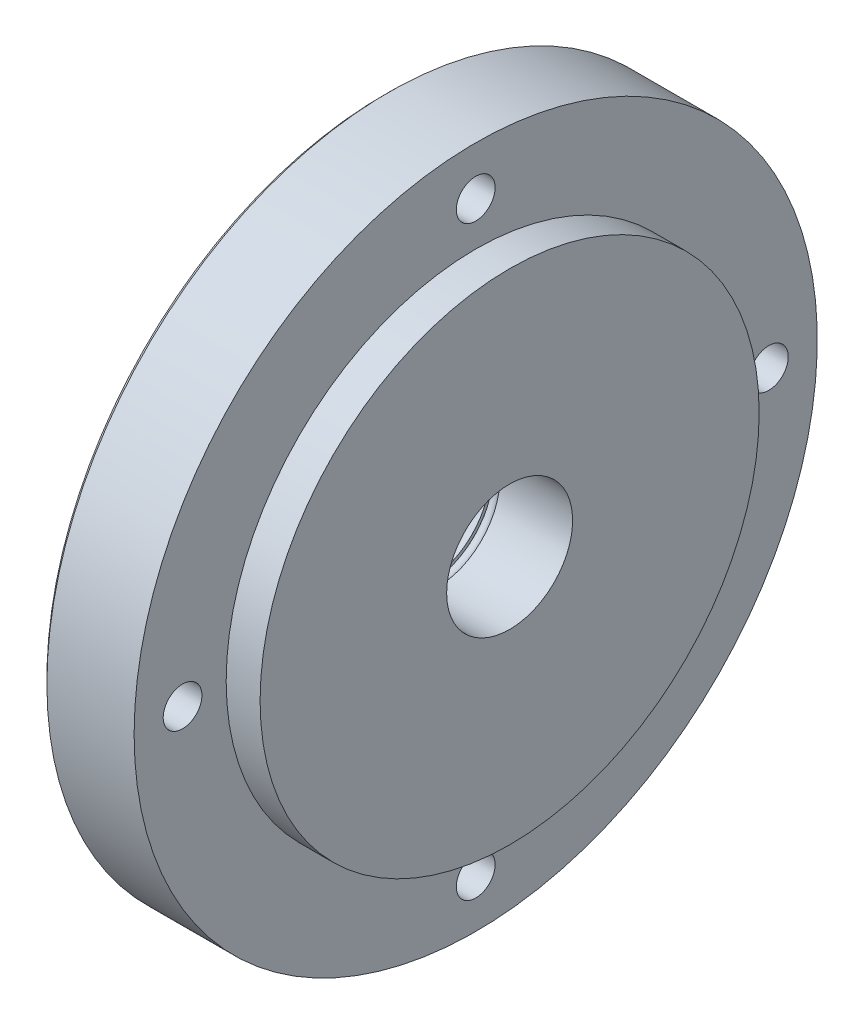
from build123d import *

# Parameters (mm, degrees)
CHAMFER1_SIZE      = 0.5
CHAMFER2_SIZE      = 1
SKETCH2_R          = 4
CUT_EXTRUDE2_DEPTH = 61
SKETCH6_R          = 7
CUT_EXTRUDE3_DEPTH = 6
SKETCH8_R          = 1
SKETCH9_R          = 4
CUT_EXTRUDE4_DEPTH = 10


with BuildPart() as part:
    # Sketch1 → Revolve1 (revolve)
    with BuildSketch(Plane.XY, mode=Mode.PRIVATE) as revolve1_sk:
        Polygon((-47.572192513, 13), (-47.572192513, 31), (-41.572192513, 31), (-41.572192513, 70.5), (-22.572192513, 70.5), (-22.572192513, 51.5), (-15.572192513, 51.5), (-15.572192513, 13), (-30.572192513, 13), (-30.572192513, 15), (-32.572192513, 15), (-32.572192513, 13), align=None)
    revolve(revolve1_sk.sketch.rotate(Axis((-70.844919786, 0, 0), (1, 0, 0)), 90), axis=Axis((-70.844919786, 0, 0), (1, 0, 0)))

    # Chamfer1
    chamfer1_edges = [part.edges().sort_by_distance(p)[0] for p in [
        (-47.572192513, 0, -31),
    ]]
    chamfer(chamfer1_edges, length=CHAMFER1_SIZE)

    # Chamfer2
    chamfer2_edges = [part.edges().sort_by_distance(p)[0] for p in [
        (-41.572192513, 0, -70.5),
    ]]
    chamfer(chamfer2_edges, length=CHAMFER2_SIZE)

    # Sketch2 → Cut-Extrude2 (cut)
    with BuildSketch(Plane.ZY.offset(41.572192513)):
        with Locations((0, -60.5)):
            Circle(SKETCH2_R)
        with Locations((-60.5, 0)):
            Circle(SKETCH2_R)
        with Locations((0, 60.5)):
            Circle(SKETCH2_R)
        with Locations((60.5, 0)):
            Circle(SKETCH2_R)
    extrude(amount=-CUT_EXTRUDE2_DEPTH, mode=Mode.SUBTRACT)

    # Sketch6 → Cut-Extrude3 (cut)
    with BuildSketch(Plane.ZY.offset(41.572192513)):
        with Locations((0, -60.5)):
            Circle(SKETCH6_R)
        with Locations((-60.5, 0)):
            Circle(SKETCH6_R)
        with Locations((60.5, 0)):
            Circle(SKETCH6_R)
        with Locations((0, 60.5)):
            Circle(SKETCH6_R)
    extrude(amount=-CUT_EXTRUDE3_DEPTH, mode=Mode.SUBTRACT)

    # Sketch9 → Cut-Extrude4 (cut)
    with BuildSketch(Plane.ZY.offset(41.572192513)):
        with Locations((42.779960262, -42.779960262)):
            Circle(SKETCH9_R)
        with Locations((42.779960262, 42.779960262)):
            Circle(SKETCH9_R)
        with Locations((-42.779960262, -42.779960262)):
            Circle(SKETCH9_R)
        with Locations((-42.779960262, 42.779960262)):
            Circle(SKETCH9_R)
    extrude(amount=-CUT_EXTRUDE4_DEPTH, mode=Mode.SUBTRACT)


with BuildPart() as body_2:
    # Sketch8 → Revolve3 (revolve)
    with BuildSketch(Plane.XY, mode=Mode.PRIVATE) as revolve3_sk:
        with Locations((-31.572192513, 14)):
            Circle(SKETCH8_R)
    revolve(revolve3_sk.sketch.rotate(Axis((-55.043716919, 0, 0), (1, 0, 0)), 270), axis=Axis((-55.043716919, 0, 0), (1, 0, 0)))


solid = Compound([part.part, body_2.part])
